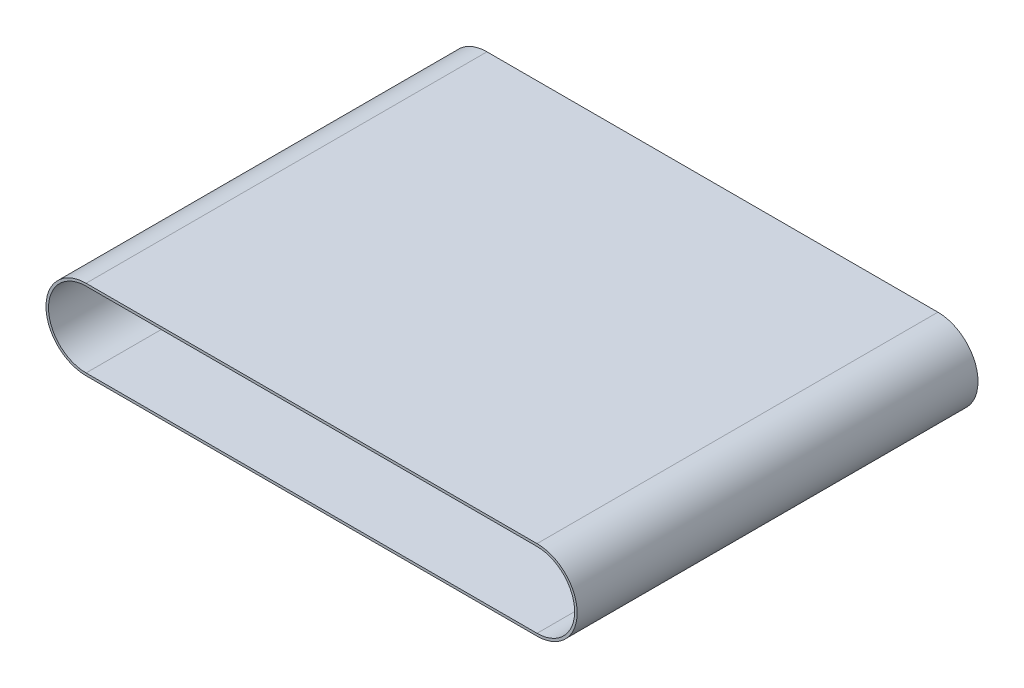
SolidWorks part; units mm, degrees
material "硅橡胶"
ref_plane "前视基准面" through (0, 0, 0) normal (0, 0, 1) x (1, 0, 0)
ref_plane "上视基准面" through (0, 0, 0) normal (0, 1, 0) x (1, 0, 0)
ref_plane "右视基准面" through (0, 0, 0) normal (1, 0, 0) x (0, 0, -1)
sketch "草图1" plane through (0, 0, 0) normal (0, 0, 1) x (1, 0, 0)
  line L1 (-450, 80.0606) -> (450, 80.0606)
  line L3 (-450, -69.9394) -> (450, -69.9394)
  line L5 (-450, 80.0606) -> (450, -69.9394) construction
  line L6 (-450, -69.9394) -> (450, 80.0606) construction
  arc A1 (-450, 80.0606) -> (-450, -69.9394) centre (-450, 5.0606) ccw
  arc A2 (450, -69.9394) -> (450, 80.0606) centre (450, 5.0606) ccw
  dimension "D2" = 75
  dimension "D1" = 900
extrude "拉伸-薄壁1" add sketch "草图1" along normal blind 800 thin contours A2 L1 A1 L3 thin type one direction wall 5
